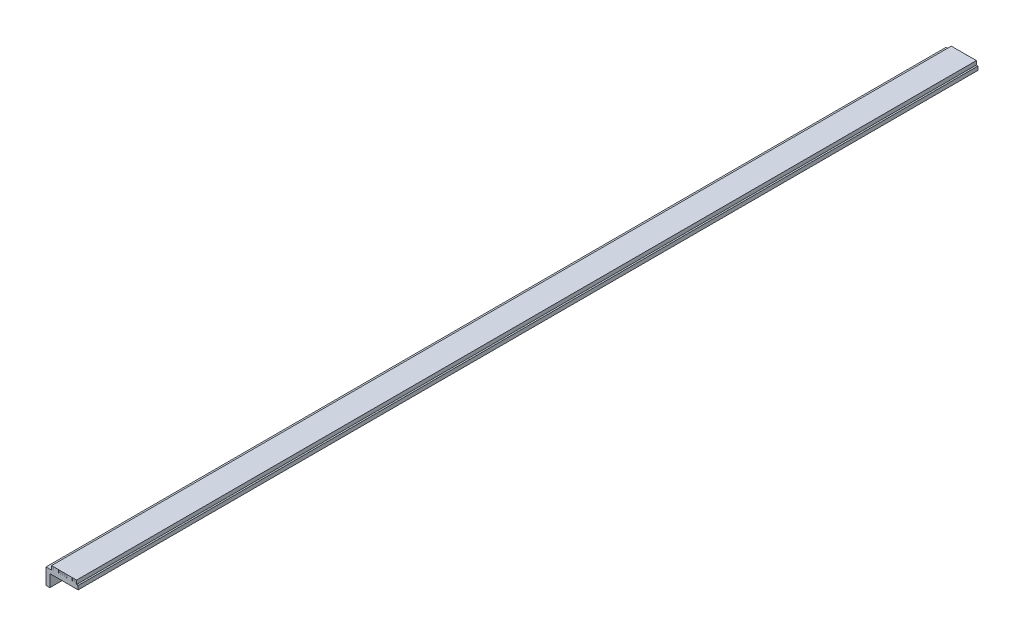
SolidWorks part; units mm, degrees
ref_plane "Front Plane" through (0, 0, 0) normal (0, 0, 1) x (1, 0, 0)
ref_plane "Top Plane" through (0, 0, 0) normal (0, 1, 0) x (1, 0, 0)
ref_plane "Right Plane" through (0, 0, 0) normal (1, 0, 0) x (0, 0, -1)
other "Configuration Table"
sketch "Sketch1" plane through (0, 0, 0) normal (0, 0, 1) x (1, 0, 0)
  line L0 (0, 0) -> (100, 0)
  line L1 (0, 0) -> (0, 100)
  line L2 (12, 12) -> (17, 12)
  line L3 (12, 12) -> (12, 100)
  line L4 (12, 100) -> (0, 100)
  line L5 (100, 12) -> (100, 0)
  line L6 (17, 12) -> (17, 24)
  line L7 (17, 24) -> (95, 24)
  line L8 (95, 24) -> (95, 12)
  line L9 (95, 12) -> (100, 12)
  line L10 (12, 12) -> (100, 12) construction
  dimension "D1" = 100
  dimension "D2" = 100
  dimension "D4" = 12
  dimension "D5" = 5
  dimension "D6" = 5
  dimension "D3" = 12
extrude "Boss-Extrude1" add sketch "Sketch1" along normal blind 2800
sketch "Sketch2" plane through (0, 0, 2800) normal (0, 0, 1) x (1, 0, 0)
  line L0 (95, 24) -> (17, 24) construction
  line L1 (21.4792, 24) -> (22.7391, 24)
  line L2 (21.4792, 24) -> (21.4792, 14.9569)
  line L3 (21.4792, 14.9569) -> (22.7391, 14.9569)
  line L4 (22.7391, 24) -> (22.7391, 14.9569)
  line L5 (21.4792, 24) -> (22.7391, 14.9569) construction
  line L6 (21.4792, 14.9569) -> (22.7391, 24) construction
  point P0 (22.1092, 19.4785)
extrude "Cut-Extrude1" cut sketch "Sketch2" against normal blind 0.2
pattern_linear "LPattern1" count 16 spacing 6 along (1, 0, 0) of "Cut-Extrude1"
ref_plane "Plane1" through (0, 0, 1400) normal (0, 0, -1) x (-1, 0, 0)
mirror "Mirror1" about plane through (0, 0, 1400) normal (0, 0, -1) of "LPattern1", "Cut-Extrude1"
sketch "Sketch3" plane through (0, 0, 2800) normal (0, 0, 1) x (1, 0, 0)
  line L1 (12, 12) -> (0, 12)
  line L2 (12, 12) -> (12, 100)
  line L3 (12, 100) -> (0, 100)
  line L4 (0, 12) -> (0, 100)
sketch "Sketch5" plane through (0, 0, 2800) normal (0, 0, 1) x (1, 0, 0)
  line L1 (0, 12) -> (12, 12)
  line L2 (0, 12) -> (0, -38)
  line L3 (0, -38) -> (12, -38)
  line L4 (12, 12) -> (12, -38)
  dimension "D1" = 50
extrude "Boss-Extrude2" add sketch "Sketch5" against normal blind 2800
extrude "Cut-Extrude3" cut sketch "Sketch3" against normal through all
